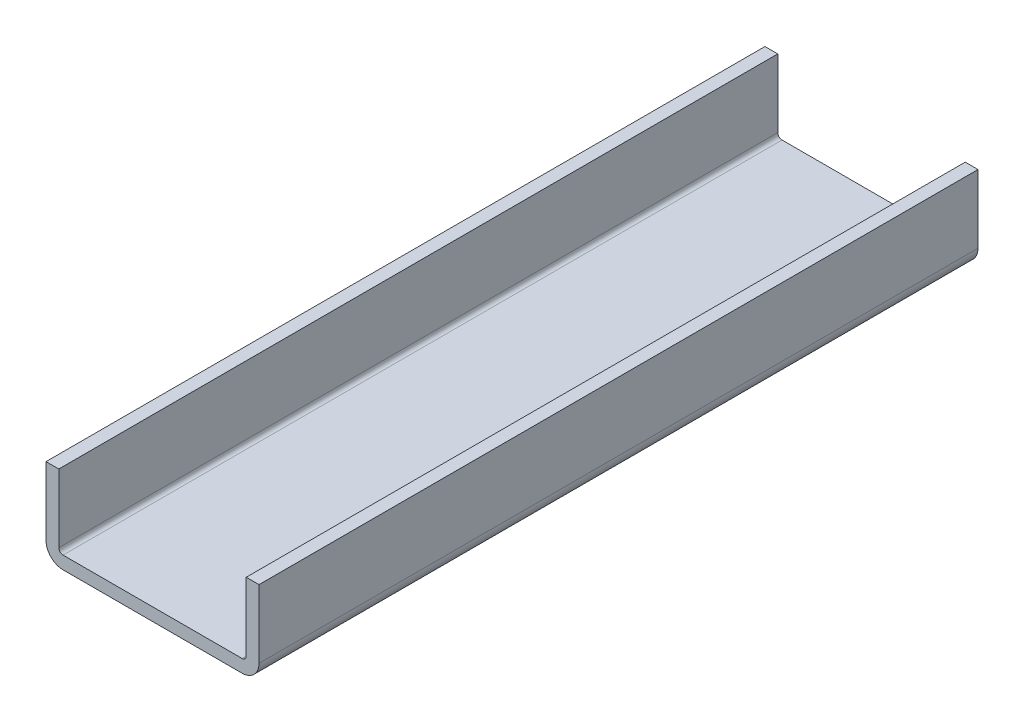
from build123d import *

# Parameters (mm, degrees)
BOSS_EXTRUDE2_DEPTH = 337.5


with BuildPart() as part:
    # Sketch2 → Boss-Extrude2 (new body)
    with BuildSketch(Plane.XY):
        with BuildLine():
            Line((0, 0), (0, -32))
            ThreePointArc((0, -32), (2.343145751, -37.656854249), (8, -40))
            Line((8, -40), (92, -40))
            ThreePointArc((92, -40), (97.656854249, -37.656854249), (100, -32))
            Line((100, -32), (100, 0))
            Line((100, 0), (94, 0))
            Line((94, 0), (94, -32))
            ThreePointArc((94, -32), (93.414213562, -33.414213562), (92, -34))
            Line((92, -34), (8, -34))
            ThreePointArc((8, -34), (6.585786438, -33.414213562), (6, -32))
            Line((6, -32), (6, 0))
            Line((6, 0), (0, 0))
        make_face()
    extrude(amount=BOSS_EXTRUDE2_DEPTH)


solid = part.part
